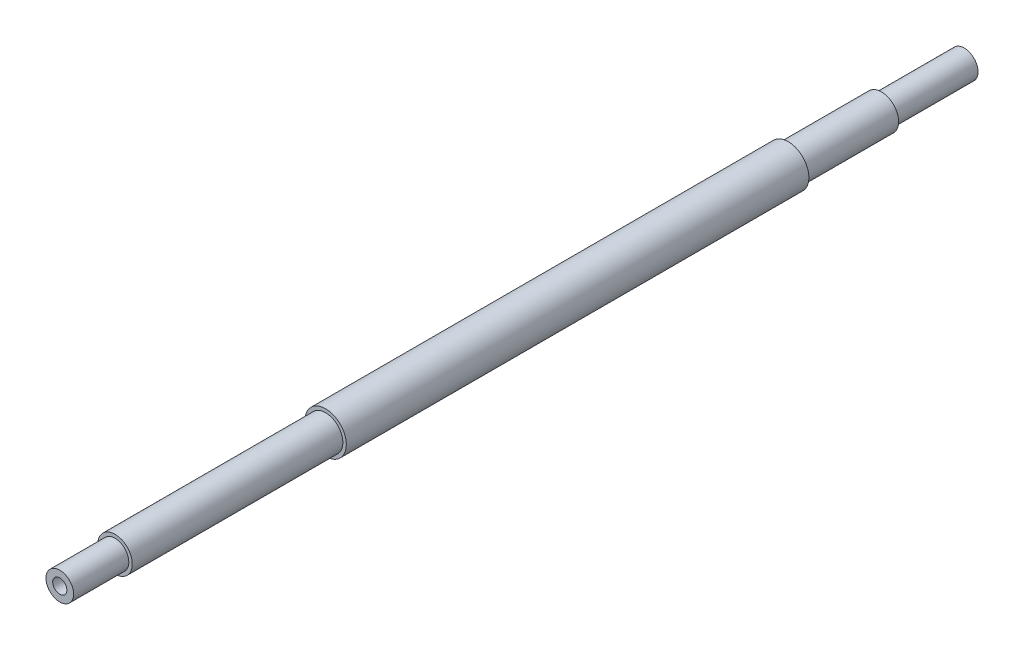
SolidWorks part; units mm, degrees
ref_plane "Front Plane" through (0, 0, 0) normal (0, 0, 1) x (1, 0, 0)
ref_plane "Top Plane" through (0, 0, 0) normal (0, 1, 0) x (1, 0, 0)
ref_plane "Right Plane" through (0, 0, 0) normal (1, 0, 0) x (0, 0, -1)
sketch "Sketch1" plane through (0, 0, 0) normal (0, 0, 1) x (1, 0, 0)
  circle A0 centre (0, 0) radius 2.5
extrude "Boss-Extrude1" add sketch "Sketch1" along normal blind 13.5
sketch "Sketch2" plane through (0, 0, 13.5) normal (0, 0, 1) x (1, 0, 0)
  circle A0 centre (0, 0) radius 3
extrude "Boss-Extrude2" add sketch "Sketch2" along normal blind 67
sketch "Sketch3" plane through (0, 0, 80.5) normal (0, 0, 1) x (1, 0, 0)
  circle A0 centre (0, 0) radius 2.5
extrude "Boss-Extrude3" add sketch "Sketch3" along normal blind 30.5
sketch "Sketch4" plane through (0, 0, 111) normal (0, 0, 1) x (1, 0, 0)
  circle A0 centre (0, 0) radius 2
extrude "Boss-Extrude4" add sketch "Sketch4" along normal blind 8
sketch "Sketch5" plane through (0, 0, 0) normal (0, 0, -1) x (-1, 0, 0)
  circle A0 centre (0, 0) radius 2
extrude "Boss-Extrude5" add sketch "Sketch5" along normal blind 12
hole_wizard "M2.5 Tapped Hole1" positions "3DSketch4" profile "Sketch9" tap size "M2.5" standard "GB"
sketch3d "3DSketch4"
  line L0 (0, 0, 119) -> (0, 0, 111) construction
  point P0 (0, 0, 119)
sketch "Sketch9" plane through (0, 0, 119) normal (1, 0, 0) x (0, -1, 0)
  line L0 (0, 0) -> (0, 6.9659)
  line L1 (0, 6.9659) -> (1.025, 6.35)
  line L2 (1.025, 6.35) -> (1.025, 0)
  line L5 (1.025, 0) -> (0, 0)
  line L10 (0, 6.9659) -> (-1.025, 6.35) construction
  line L11 (0, -6.35) -> (0, 107.95) construction
  dimension "螺纹孔钻头直径" = 2.05
  dimension "螺纹孔钻头深度" = 6.35
  dimension "导头角度" = 118
cosmetic thread "CosmeticThread1" parameters "D1"=5, "D2"=2.5
